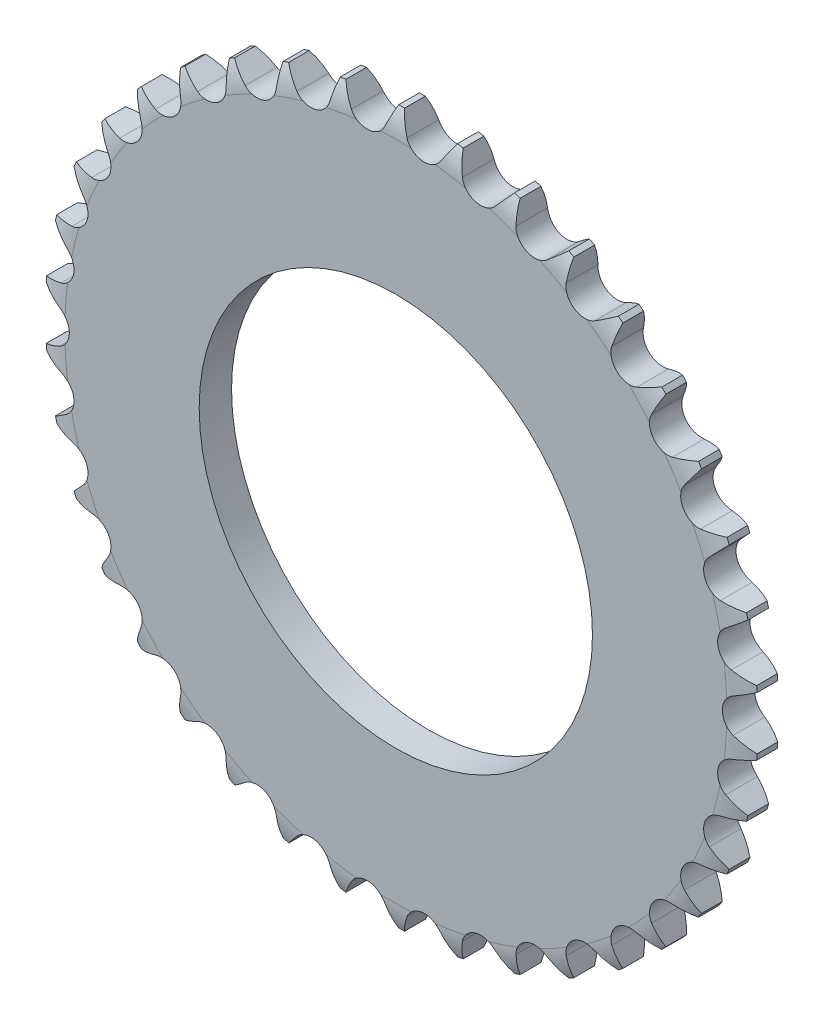
SolidWorks part; units mm, degrees
ref_plane "前视基准面" through (0, 0, 0) normal (0, 0, 1) x (1, 0, 0)
ref_plane "上视基准面" through (0, 0, 0) normal (0, 1, 0) x (1, 0, 0)
ref_plane "右视基准面" through (0, 0, 0) normal (1, 0, 0) x (0, 0, -1)
sketch "草图1" plane through (0, 0, 0) normal (1, 0, 0) x (0, 0, -1)
  line L0 (0, 0) -> (-35, 0) construction
  line L1 (0, 0) -> (0, 45)
  line L2 (0, 45) -> (-27.8, 45)
  line L3 (-35, 8) -> (0, 8)
  line L4 (-29.1, 79.3) -> (-35, 79.3)
  line L5 (-35, 79.3) -> (-35, 0)
  line L6 (-35, 76.9) -> (-27.8, 76.9) construction
  line L8 (-31.4, 76.9) -> (-31.4, 79.3) construction
  line L9 (-27.8, 76.9) -> (-27.8, 45)
  line L10 (-28, 45) -> (-28, 76.9)
  arc A0 (-27.8, 73.6334) -> (-29.1, 79.3) centre (-40.8, 73.6334) ccw
  arc A1 (-28, 73.6334) -> (-29.3, 79.3) centre (-41, 73.6334) ccw
  point P14 (-35, 19)
  point P15 (-28, 45)
  point P17 (-14, 45)
  point P18 (-0.1, 45)
  dimension "D1" = 16
  dimension "r" = 13
  dimension "D3" = 13
  dimension "B1" = 7.2
  dimension "D2" = 1.3
  dimension "A" = 35
  dimension "de" = 158.6
  dimension "Dp" = 153.8
  dimension "Dm" = 90
  dimension "C" = 1.3
  dimension "Z" = 38
  dimension "(b1)" = 7
  dimension "B2" = 21
  dimension "B3" = 34.9
sketch "草图3" plane through (0, 0, 0) normal (0, 0, 1) x (1, 0, 0)
  line L0 (0, 0) -> (0, 79.3) construction
  line L1 (0, 0) -> (6.35, 76.6374) construction
  line L2 (0.65, 79.2973) -> (2.4165, 75.0148)
  line L3 (0, 72.8939) -> (11.9973, 71.8999) construction
  line L4 (9.9628, 74.3896) -> (12.4101, 78.3229)
  line L5 (-0.65, 79.2973) -> (-2.4165, 75.0148) construction
  line L6 (0, 79.3) -> (0, 0) construction
  circle A0 centre (0, 0) radius 79.3 construction
  circle A1 centre (6.35, 76.6374) radius 4.255
  circle A2 centre (-6.35, 76.6374) radius 4.255 construction
  circle A3 centre (0, 0) radius 81.155 construction
  point P13 (-12.4101, 78.3229)
  point P15 (5.9986, 72.3969)
  dimension "D1" = 8.51
  dimension "D3" = 162.31
  dimension "D4" = 1.3
  dimension "D2" = 12.7
sketch "草图4" plane through (0, 0, 0) normal (1, 0, 0) x (0, 0, -1)
  line L0 (-35, 43.75) -> (-27.8, 43.75)
  line L1 (-31.4, 76.9) -> (-31.4, 79.3) construction
  line L2 (-31.4, 76.9) -> (-31.4, 79.3) construction
  line L8 (-35, 79.3) -> (-35, 0) construction
  line L9 (-29.1, 79.3) -> (-35, 79.3) construction
  line L10 (-27.8, 76.9) -> (-27.8, 45) construction
  line L14 (-35, 73.6334) -> (-35, 43.75)
  line L15 (-29.1, 79.3) -> (-33.7, 79.3)
  line L16 (-27.8, 73.6334) -> (-27.8, 43.75)
  arc A0 (-35, 73.6334) -> (-33.7, 79.3) centre (-22, 73.6334) cw
  arc A1 (-27.8, 73.6334) -> (-29.1, 79.3) centre (-40.8, 73.6334) ccw construction
  arc A2 (-27.8, 73.6334) -> (-29.1, 79.3) centre (-40.8, 73.6334) ccw
  dimension "D1" = 43.75
revolve "旋转1" add sketch "草图4" angle 360 about L0
sketch "草图5" plane through (0, 0, 0) normal (0, 0, 1) x (1, 0, 0)
  line L0 (0.65, 79.2973) -> (2.4165, 75.0148) construction
  line L1 (9.9628, 74.3896) -> (12.4101, 78.3229) construction
  line L2 (0.65, 79.2973) -> (2.4165, 75.0148)
  line L3 (9.9628, 74.3896) -> (12.4101, 78.3229)
  circle A0 centre (6.35, 76.6374) radius 4.255 construction
  arc A1 (2.4165, 75.0148) -> (9.9628, 74.3896) centre (6.35, 76.6374) ccw
  circle A2 centre (0, 0) radius 79.3 construction
  arc A3 (12.4101, 78.3229) -> (0.65, 79.2973) centre (0, 0) ccw
extrude "切除-拉伸1" cut sketch "草图5" along normal through all
pattern_circular "阵列(圆周)1" count 38 over 360 about axis through (0, 0, 0) along (0, 0, 1) of "切除-拉伸1"
sketch "草图9" [suppressed] plane through (0, 0, 0) normal (1, 0, 0) x (0, 0, -1)
  line L1 (-34.1, 71.25) -> (-40, 71.25) construction
  line L5 (-40, 71.25) -> (-40, 0) construction
  line L6 (-33, 50) -> (-33, 68.82) construction
  line L7 (-34.3, 71.25) -> (-38.7, 71.25)
  line L8 (-40, 65.5834) -> (-40, 50)
  line L10 (-33, 50) -> (-33, 65.5834)
  line L11 (-33, 65.5834) -> (-40, 65.5834) construction
  line L12 (-36.5, 65.5834) -> (-36.5, 71.25) construction
  line L14 (-33, 50) -> (-40, 50)
  arc A0 (-33, 65.5834) -> (-34.3, 71.25) centre (-46, 65.5834) ccw construction
  arc A1 (-33, 65.5834) -> (-34.3, 71.25) centre (-46, 65.5834) ccw
  arc A2 (-40, 65.5834) -> (-38.7, 71.25) centre (-27, 65.5834) cw
revolve "旋转3" [suppressed] add sketch "草图9" angle 360 about L0
sketch "草图10" [suppressed] plane through (0, 0, 0) normal (1, 0, 0) x (0, 0, -1)
  line L0 (0, 50) -> (-32.8, 50) construction
  line L1 (0, 50) -> (-40, 50)
  line L2 (0, 0) -> (0, 50) construction
  line L3 (-40, 10) -> (0, 10) construction
  line L4 (0, 10) -> (0, 50)
  line L5 (-40, 10) -> (0, 10)
  line L6 (-33, 50) -> (-33, 10) construction
  line L7 (-40, 71.25) -> (-40, 0) construction
  line L11 (-40, 50) -> (-40, 10)
revolve "旋转4" [suppressed] add sketch "草图10" angle 360 about L0
sketch "草图8" [suppressed] plane through (0, 0, 0) normal (0, 0, 1) x (1, 0, 0)
  line L0 (0.65, 71.247) -> (2.4085, 66.9233) construction
  line L1 (9.9298, 66.2264) -> (12.4529, 70.1533) construction
  line L2 (0.65, 71.247) -> (2.4085, 66.9233)
  line L3 (9.9298, 66.2264) -> (12.4529, 70.1533)
  circle A0 centre (6.35, 68.5264) radius 4.255 construction
  arc A1 (2.4085, 66.9233) -> (9.9298, 66.2264) centre (6.35, 68.5264) ccw
  circle A2 centre (0, 0) radius 71.25 construction
  arc A3 (12.4529, 70.1533) -> (0.65, 71.247) centre (0, 0) ccw
extrude "切除-拉伸3" [suppressed] cut sketch "草图8" along normal through all
pattern_circular "阵列(圆周)3" [suppressed] count 38 over 360
pattern_linear "阵列(线性)7" [suppressed] count 2 spacing 14 along (0, 0, 1)
sketch "草图15" [suppressed] plane through (0, 0, 0) normal (0, 0, -1) x (-1, 0, 0)
  line L0 (0, 10) -> (0, 50) construction
  circle A1 centre (0, 0) radius 30 construction
  text T0 "xxxxxxxxxxxx    电话：xxxxxxxxxxxx    网址：xxxxxxxxxxxxxx\r\n" font "Century Gothic" height 0.8
  point P1 (0, 30)
extrude "LOGO2" [suppressed] cut sketch "草图15" against normal blind 0.001
sketch "草图11" [suppressed] plane through (0, 0, 0) normal (1, 0, 0) x (0, 0, -1)
  line L0 (-55, 83.35) -> (-55, 0) construction
  line L1 (-55, 83.35) -> (-55, 12.5) construction
  line L2 (-49.1, 83.35) -> (-55, 83.35) construction
  line L3 (0, 60) -> (-47.8, 60) construction
  line L4 (-48, 70.4675) -> (-55, 70.4675) construction
  line L5 (0, 0) -> (0, 60) construction
  line L7 (-49.1, 83.35) -> (-55, 83.35) construction
  line L8 (-51.5, 70.4675) -> (-51.5, 83.35) construction
  line L9 (-55, 12.5) -> (0, 12.5) construction
  line L10 (0, 12.5) -> (0, 60) construction
  line L11 (-55, 12.5) -> (0, 12.5)
  line L16 (-48, 60) -> (-48, 77.6834) construction
  line L17 (0, 60) -> (0, 12.5)
  line L18 (-48, 60) -> (-48, 80.935) construction
  line L23 (-55, 60) -> (-55, 12.5)
  line L25 (0, 60) -> (-55, 60)
  arc A3 (-48, 77.6834) -> (-49.3, 83.35) centre (-61, 77.6834) ccw construction
  arc A5 (-48, 77.6834) -> (-49.3, 83.35) centre (-61, 77.6834) ccw construction
revolve "旋转5" [suppressed] add sketch "草图11" angle 360 about L0
sketch "草图12" [suppressed] plane through (0, 0, 0) normal (1, 0, 0) x (0, 0, -1)
  line L0 (-48, 60) -> (-48, 80.935) construction
  line L1 (-48, 77.6834) -> (-55, 77.6834) construction
  line L2 (-49.1, 83.35) -> (-55, 83.35) construction
  line L3 (-55, 83.35) -> (-55, 0) construction
  line L5 (-48, 60) -> (-48, 77.6834)
  line L6 (-51.5, 77.6834) -> (-51.5, 83.35) construction
  line L7 (-48, 60) -> (-55, 60)
  line L8 (-49.3, 83.35) -> (-53.7, 83.35)
  line L9 (-55, 77.6834) -> (-55, 60)
  arc A0 (-48, 77.6834) -> (-49.3, 83.35) centre (-61, 77.6834) ccw construction
  arc A1 (-55, 77.6834) -> (-53.7, 83.35) centre (-42, 77.6834) cw
  arc A3 (-48, 77.6834) -> (-49.3, 83.35) centre (-61, 77.6834) ccw
revolve "旋转6" [suppressed] add sketch "草图12" angle 360 about L0
sketch "草图13" [suppressed] plane through (0, 0, 0) normal (0, 0, 1) x (1, 0, 0)
  line L0 (0.65, 83.3475) -> (2.4162, 79.0636) construction
  line L1 (0.65, 83.3475) -> (2.4162, 79.0636)
  line L2 (9.9816, 78.4682) -> (12.3962, 82.423) construction
  line L3 (9.9816, 78.4682) -> (12.3962, 82.423)
  circle A0 centre (6.35, 80.6855) radius 4.255 construction
  arc A1 (2.4162, 79.0636) -> (9.9816, 78.4682) centre (6.35, 80.6855) ccw
  circle A2 centre (0, 0) radius 83.35 construction
  arc A3 (12.3962, 82.423) -> (0.65, 83.3475) centre (0, 0) ccw
extrude "切除-拉伸4" [suppressed] cut sketch "草图13" along normal through all
pattern_circular "阵列(圆周)4" [suppressed] count 38 over 360
pattern_linear "阵列(线性)9" [suppressed] count 3 spacing 13.95 along (0, 0, 1)
sketch "草图16" [suppressed] plane through (0, 0, 0) normal (0, 0, -1) x (-1, 0, 0)
  line L0 (0, 60) -> (0, 12.5) construction
  circle A1 centre (0, 0) radius 36.25 construction
  text T0 "xxxxxxxxxxxx    电话：xxxxxxxxxxxx    网址：xxxxxxxxxxxxxx\r\n" font "Century Gothic" height 0.6
  point P1 (0, 36.25)
extrude "LOGO3" [suppressed] cut sketch "草图16" against normal blind 0.001
ref_plane "基准面1" through (0, 0, 31.4) normal (0, 0, -1) x (-1, 0, 0)
